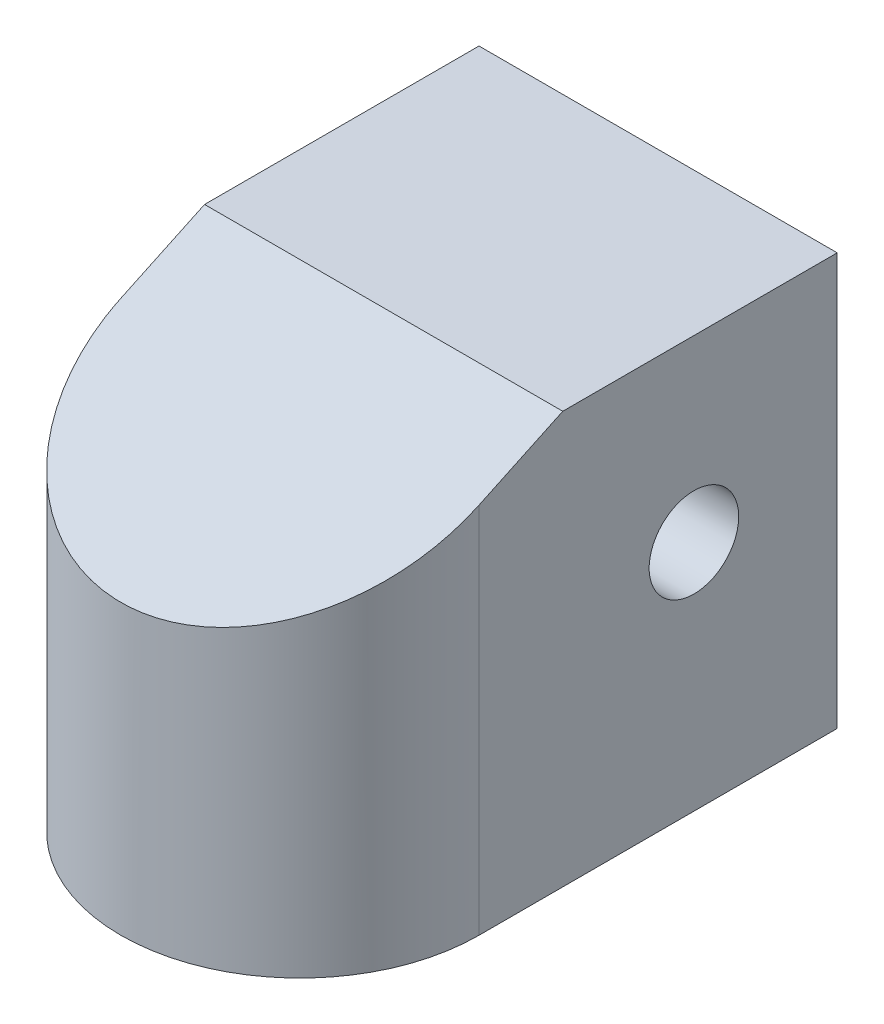
from build123d import *

# Parameters (mm, degrees)
EXTRUDE_1_DEPTH     = 23
SKETCH_2_R          = 2.5
CUT_EXTRUDE_1_DEPTH = 12
SKETCH_3_R          = 2.5
CUT_EXTRUDE_2_DEPTH = 62
CUT_EXTRUDE_3_DEPTH = 26


with BuildPart() as part:
    # 草图1 → 凸台-拉伸1 (new body)
    with BuildSketch(Plane(origin=(0, 0, 0), x_dir=(1, 0, 0), z_dir=(0, 1, 0))):
        with BuildLine():
            Line((-10, 0), (-10, 20))
            Line((-10, 20), (10, 20))
            Line((10, 20), (10, 0))
            ThreePointArc((10, 0), (0, -10), (-10, 0))
        make_face()
    extrude(amount=EXTRUDE_1_DEPTH)

    # 草图2 → 切除-拉伸1 (cut)
    with BuildSketch(Plane.XZ):
        with Locations(Location((0, 0, 0), (0, 0, 270))):
            Circle(SKETCH_2_R)
    extrude(amount=-CUT_EXTRUDE_1_DEPTH, mode=Mode.SUBTRACT)

    # 草图3 → 切除-拉伸2 (cut)
    with BuildSketch(Plane(origin=(10, 0, 0), x_dir=(0, 0, -1), z_dir=(1, 0, 0))):
        with Locations((12, 13)):
            Circle(SKETCH_3_R)
    extrude(amount=-CUT_EXTRUDE_2_DEPTH, mode=Mode.SUBTRACT)

    # 草图4 → 切除-拉伸3 (cut)
    with BuildSketch(Plane(origin=(10, 0, 0), x_dir=(0, 0, -1), z_dir=(1, 0, 0))):
        Polygon((0, 23), (-10, 23), (-10, 16.096925585), (4.676984075, 23), align=None)
    extrude(amount=-CUT_EXTRUDE_3_DEPTH, mode=Mode.SUBTRACT)


solid = part.part
